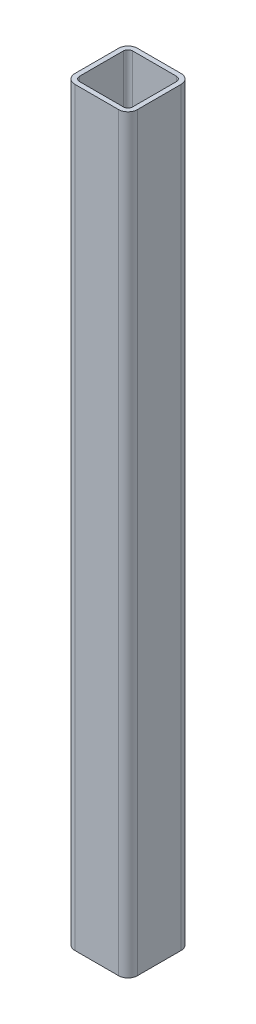
SolidWorks part; units mm, degrees
material "Q235B"
ref_plane "Front Plane" through (0, 0, 0) normal (0, 0, 1) x (1, 0, 0)
ref_plane "Top Plane" through (0, 0, 0) normal (0, 1, 0) x (1, 0, 0)
ref_plane "Right Plane" through (0, 0, 0) normal (1, 0, 0) x (0, 0, -1)
sketch "Sketch1" plane through (0, 0, 0) normal (0, 0, 1) x (1, 0, 0)
  line L0 (0, 0) -> (0, 480)
  dimension "D1" = 480
other "Cold-formed hollow square steel (gb t6728-2002) 40×3-example.com(1)"
ref_plane "Plane1" through (0, 0, 0) normal (0, 1, 0) x (-1, 0, 0)
sketch "Sketch12" plane through (0, 0, 0) normal (0, 1, 0) x (-1, 0, 0)
  line L0 (-14, -17) -> (14, -17)
  line L1 (-17, -14) -> (-17, 14)
  line L2 (14, 17) -> (-14, 17)
  line L3 (17, 14) -> (17, -14)
  line L4 (-14, -20) -> (14, -20)
  line L5 (-20, -14) -> (-20, 14)
  line L6 (14, 20) -> (-14, 20)
  line L7 (20, 14) -> (20, -14)
  arc A0 (20, 14) -> (14, 20) centre (14, 14) ccw
  arc A1 (14, -20) -> (20, -14) centre (14, -14) ccw
  arc A2 (-20, -14) -> (-14, -20) centre (-14, -14) ccw
  arc A3 (-14, 20) -> (-20, 14) centre (-14, 14) ccw
  arc A4 (-14, 17) -> (-17, 14) centre (-14, 14) ccw
  arc A5 (17, 14) -> (14, 17) centre (14, 14) ccw
  arc A6 (14, -17) -> (17, -14) centre (14, -14) ccw
  arc A7 (-17, -14) -> (-14, -17) centre (-14, -14) ccw
  point P0 (-20, 0)
  point P1 (20, 0)
  point P2 (0, 20)
  point P3 (0, -20)
  point P4 (0, 0)
  point P5 (-20, -20)
  point P6 (20, -20)
  point P7 (20, 20)
  point P8 (-20, 20)
  point P33 (0, 0)
  dimension "D1" = 6
  dimension "D2" = 40
  dimension "D3" = 3
